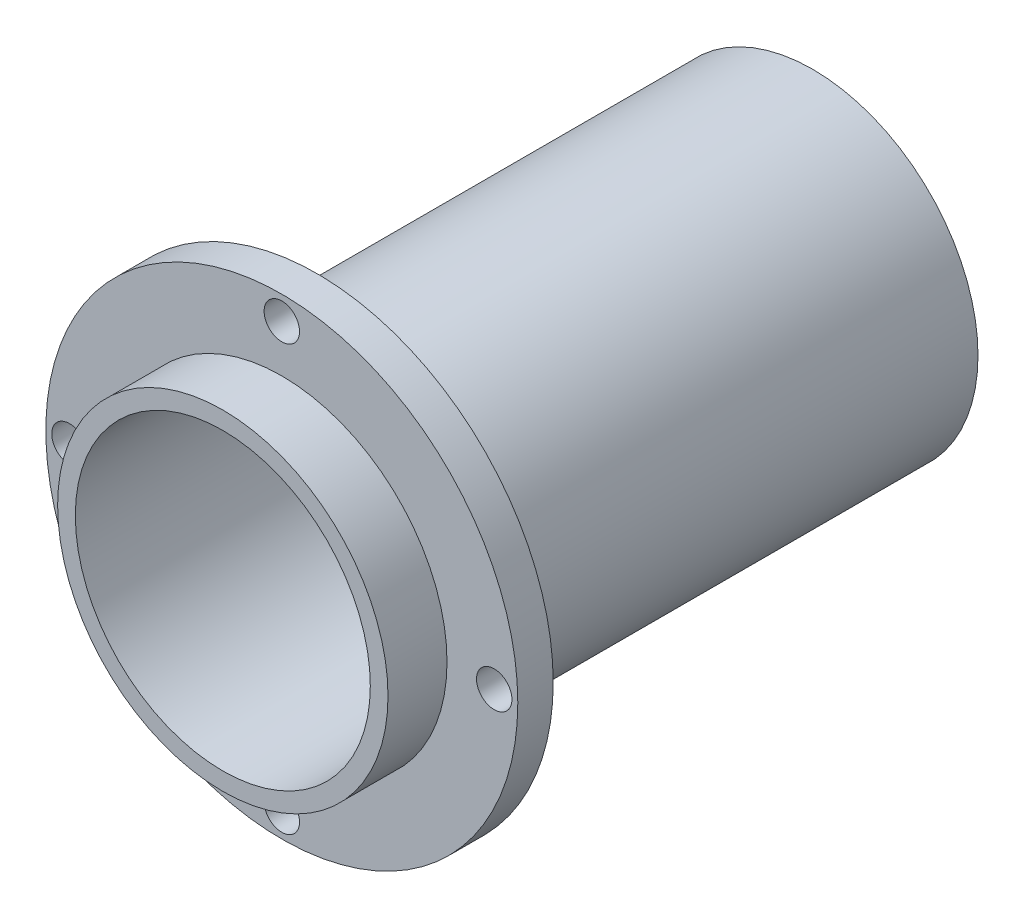
SolidWorks part; units mm, degrees
ref_plane "Front Plane" through (0, 0, 0) normal (0, 0, 1) x (1, 0, 0)
ref_plane "Top Plane" through (0, 0, 0) normal (0, 1, 0) x (1, 0, 0)
ref_plane "Right Plane" through (0, 0, 0) normal (1, 0, 0) x (0, 0, -1)
sketch "Sketch1" plane through (0, 0, 0) normal (0, 0, 1) x (1, 0, 0)
  circle A0 centre (0, 0) radius 14
  circle A1 centre (0, 0) radius 12.5
  dimension "D1" = 28
  dimension "D2" = 1.5
extrude "Boss-Extrude1" add sketch "Sketch1" along normal mid plane 50
sketch "Sketch2" plane through (0, 0, 25) normal (0, 0, 1) x (1, 0, 0)
  circle A0 centre (0, 0) radius 20
  circle A1 centre (0, 18) radius 1.5
  circle A2 centre (18, 0) radius 1.5
  circle A3 centre (0, -18) radius 1.5
  circle A4 centre (-18, 0) radius 1.5
  circle A5 centre (0, 0) radius 12.5
  point P14 (0, 0)
  dimension "D1" = 18
  dimension "D2" = 40
  dimension "D3" = 3
  dimension "D4" = 4
extrude "Boss-Extrude2" add sketch "Sketch2" against normal blind 3 from offset 5
